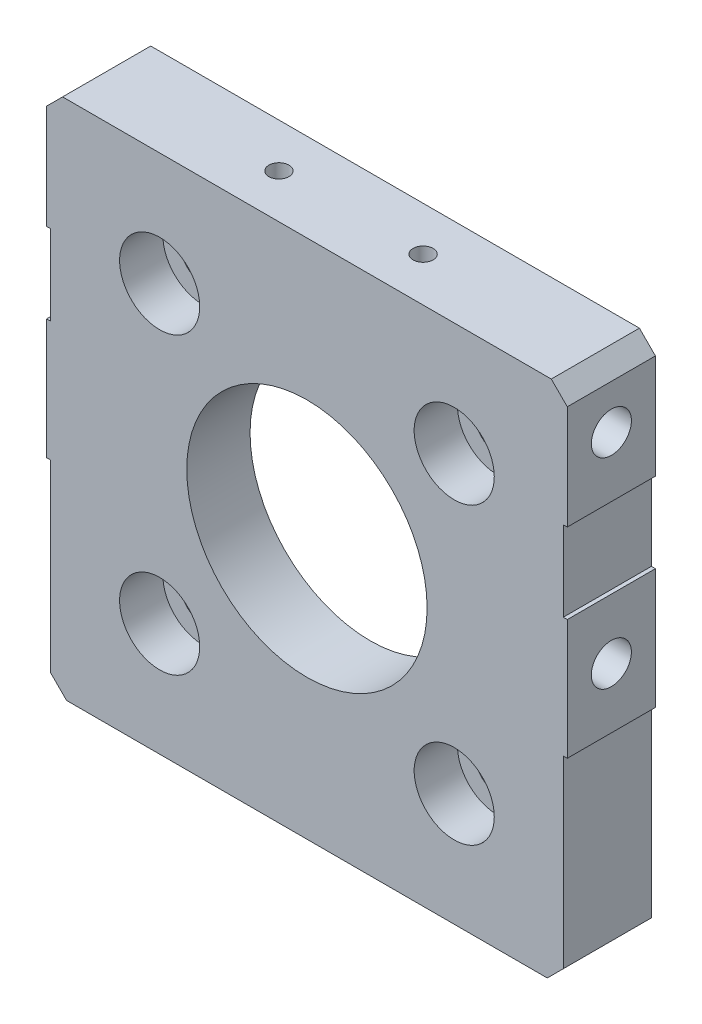
SolidWorks part; units mm, degrees
material "SUS304"
ref_plane "前视基准面" through (0, 0, 0) normal (0, 0, 1) x (1, 0, 0)
ref_plane "上视基准面" through (0, 0, 0) normal (0, 1, 0) x (1, 0, 0)
ref_plane "右视基准面" through (0, 0, 0) normal (1, 0, 0) x (0, 0, -1)
sketch "草图1" plane through (0, 0, 0) normal (0, 0, 1) x (1, 0, 0)
  line L1 (-32.5, -32.5) -> (32.5, -32.5)
  line L2 (-32.5, -32.5) -> (-32.5, 32.5)
  line L3 (-32.5, 32.5) -> (32.5, 32.5)
  line L4 (32.5, -32.5) -> (32.5, 32.5)
  line L5 (-32.5, -32.5) -> (32.5, 32.5) construction
  line L6 (-32.5, 32.5) -> (32.5, -32.5) construction
  point P0 (0, 0)
  dimension "D1" = 65
  dimension "D2" = 65
extrude "凸台-拉伸1" add sketch "草图1" along normal mid plane 11
sketch "草图3" plane through (0, 0, -5.5) normal (0, 0, -1) x (-1, 0, 0)
  circle A0 centre (0, 0) radius 20.05
  dimension "D1" = 40.1
extrude "切除-拉伸1" cut sketch "草图3" against normal blind 3.1
sketch "草图4" plane through (0, 0, -2.4) normal (0, 0, -1) x (-1, 0, 0)
  circle A0 centre (0, 0) radius 15
  dimension "D1" = 30
extrude "切除-拉伸2" cut sketch "草图4" against normal through all
hole_wizard "M5 六角凹头螺钉的柱形沉头孔1" positions "草图6" profile "草图5" counterbore size "M5" standard "ISO" end condition through all
sketch "草图6" plane through (0, 0, 5.5) normal (0, 0, 1) x (1, 0, 0)
  point P0 (-18.3848, 18.3848)
  point P3 (18.3848, 18.3848)
  point P6 (18.3848, -18.3848)
  point P9 (-18.3848, -18.3848)
sketch "草图5" plane through (-18.3848, 18.3848, 5.5) normal (1, 0, 0) x (0, -1, 0)
  line L0 (0, 0) -> (0, 11)
  line L1 (0, 11) -> (2.75, 11)
  line L3 (2.75, 11) -> (2.75, 5.4)
  line L4 (2.75, 5.4) -> (5, 5.4)
  line L5 (5, 5.4) -> (5, 0)
  line L7 (5, 0) -> (0, 0)
  line L11 (0, -6.35) -> (0, 107.95) construction
  dimension "通孔孔直径" = 5.5
  dimension "通孔孔深度" = 11
  dimension "柱形沉头孔直径" = 10
  dimension "柱形沉头孔深度" = 5.4
sketch "草图7" plane through (-32.5, 0, 0) normal (-1, 0, 0) x (0, 0, 1)
  circle A0 centre (0, 25) radius 4
  dimension "D1" = 8
  dimension "D2" = 25
extrude "凸台-拉伸2" [suppressed] add sketch "草图7" along normal blind 5
hole_wizard "M6 螺纹孔1" positions "草图9" profile "草图8" tap size "M6" standard "GB"
sketch "草图9" plane through (-32.5, 0, 0) normal (-1, 0, 0) x (0, 0, 1)
  point P0 (0, 0)
  point P4 (0, 25)
  dimension "D1" = 25
sketch "草图8" plane through (-32.5, 0, 0) normal (0, 1, 0) x (0, 0, 1)
  line L0 (0, 0) -> (0, 11.5022)
  line L1 (0, 11.5022) -> (2.5, 10)
  line L2 (2.5, 10) -> (2.5, 0)
  line L5 (2.5, 0) -> (0, 0)
  line L10 (0, 11.5022) -> (-2.5, 10) construction
  line L11 (0, -6.35) -> (0, 107.95) construction
  dimension "螺纹孔钻头直径" = 5
  dimension "螺纹孔钻头深度" = 10
  dimension "导头角度" = 118
cosmetic thread "孔螺蚊线1" parameters "D1"=10, "D2"=6
cosmetic thread "孔螺蚊线3" parameters "D1"=10, "D2"=6
sketch "草图12" plane through (-32.5, 0, 0) normal (-1, 0, 0) x (0, 0, 1)
  line L0 (-5.5, 32.5) -> (-5.5, -32.5) construction
  line L1 (-5.5, 17.5) -> (5.5, 17.5)
  line L2 (-5.5, 17.5) -> (-5.5, 7.5)
  line L3 (-5.5, 7.5) -> (5.5, 7.5)
  line L4 (5.5, 17.5) -> (5.5, 7.5)
  line L5 (5.5, 32.5) -> (5.5, -32.5) construction
  line L7 (-5.5, -7.5) -> (5.5, -7.5)
  line L8 (-5.5, -7.5) -> (-5.5, -32.5)
  line L9 (-5.5, -32.5) -> (5.5, -32.5)
  line L10 (5.5, -7.5) -> (5.5, -32.5)
  circle A0 centre (0, 25) radius 2.5 construction
  dimension "D1" = 7.5
  dimension "D2" = 7.5
  dimension "D3" = 7.5
extrude "切除-拉伸3" cut sketch "草图12" against normal blind 0.5
mirror "镜向1" about plane through (0, 0, 0) normal (1, 0, 0) of "切除-拉伸3", "M6 螺纹孔1"
hole_wizard "M3 螺纹孔1" positions "草图14" profile "草图13" tap size "M3" standard "GB"
sketch "草图14" plane through (0, -32.5, 0) normal (0, -1, 0) x (-1, 0, 0)
  line L0 (-32, 6) -> (-32, -6) construction
  point P0 (-14, 0)
  point P2 (-6, 0)
  dimension "D1" = 18
  dimension "D2" = 8
sketch "草图13" plane through (14, -32.5, 0) normal (1, 0, 0) x (0, 0, -1)
  line L0 (0, 0) -> (0, 11.2511)
  line L1 (0, 11.2511) -> (1.25, 10.5)
  line L2 (1.25, 10.5) -> (1.25, 0)
  line L5 (1.25, 0) -> (0, 0)
  line L10 (0, 11.2511) -> (-1.25, 10.5) construction
  line L11 (0, -6.35) -> (0, 107.95) construction
  dimension "螺纹孔钻头直径" = 2.5
  dimension "螺纹孔钻头深度" = 10.5
  dimension "导头角度" = 118
cosmetic thread "孔螺蚊线4" [suppressed] parameters "D1"=8, "D2"=3
cosmetic thread "孔螺蚊线5" [suppressed] parameters "D1"=8, "D2"=3
chamfer "倒角1" distance 2 angle 45 4 edges at (-32.5, 32.5, 0) (32.5, 32.5, 0) (-32, -32.5, 0) (32, -32.5, 0)
hole_wizard "M3 螺纹孔2" positions "草图15" profile "草图16" tap size "M3" standard "ISO"
sketch "草图15" plane through (0, 32.5, 0) normal (0, 1, 0) x (1, 0, 0)
  line L3 (30.5, 0) -> (-30.5, 0) construction
  line L4 (30.5, -5.5) -> (30.5, 5.5) construction
  line L5 (-30.5, 5.5) -> (-30.5, -5.5) construction
  line L6 (0, 5.5) -> (0, -5.5) construction
  line L7 (30.5, 5.5) -> (-30.5, 5.5) construction
  line L8 (30.5, -5.5) -> (-30.5, -5.5) construction
  point P22 (-9, 0)
  point P36 (9, 0)
  dimension "D1" = 18
sketch "草图16" plane through (-9, 32.5, 0) normal (1, 0, 0) x (0, 0, 1)
  line L0 (0, 0) -> (0, 9.2511)
  line L1 (0, 9.2511) -> (1.25, 8.5)
  line L2 (1.25, 8.5) -> (1.25, 0)
  line L5 (1.25, 0) -> (0, 0)
  line L10 (0, 9.2511) -> (-1.25, 8.5) construction
  line L11 (0, -6.35) -> (0, 107.95) construction
  dimension "螺纹孔钻头直径" = 2.5
  dimension "螺纹孔钻头深度" = 8.5
  dimension "导头角度" = 118
cosmetic thread "孔螺蚊线10" parameters "D1"=6, "D2"=3
cosmetic thread "孔螺蚊线11" parameters "D1"=6, "D2"=3
hole_wizard "M3 螺纹孔3" positions "草图17" profile "草图18" tap size "M3" standard "ISO"
sketch "草图17" plane through (0, -32.5, 0) normal (0, -1, 0) x (-1, 0, 0)
  line L0 (-9, 2.75) -> (-9, -0.25) construction
  line L2 (9, 2.75) -> (9, -0.25) construction
  arc A0 (-7.25, 1) -> (-10.75, 1) centre (-9, 1) ccw construction
  arc A1 (-10.75, -2) -> (-7.25, -2) centre (-9, -2) ccw construction
  arc A2 (10.75, 1) -> (7.25, 1) centre (9, 1) ccw construction
  arc A3 (7.25, -2) -> (10.75, -2) centre (9, -2) ccw construction
  point P0 (-9, 1.25)
  point P2 (9, 1.25)
sketch "草图18" plane through (9, -32.5, -1.25) normal (1, 0, 0) x (0, 0, -1)
  line L0 (0, 0) -> (0, 9.2511)
  line L1 (0, 9.2511) -> (1.25, 8.5)
  line L2 (1.25, 8.5) -> (1.25, 0)
  line L5 (1.25, 0) -> (0, 0)
  line L10 (0, 9.2511) -> (-1.25, 8.5) construction
  line L11 (0, -6.35) -> (0, 107.95) construction
  dimension "螺纹孔钻头直径" = 2.5
  dimension "螺纹孔钻头深度" = 8.5
  dimension "导头角度" = 118
cosmetic thread "孔螺蚊线12" parameters "D1"=6, "D2"=3
cosmetic thread "孔螺蚊线13" parameters "D1"=6, "D2"=3
